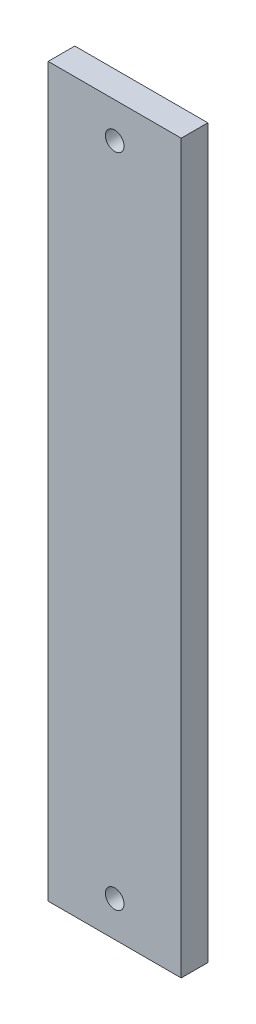
from build123d import *

# Parameters (mm, degrees)
SKETCH1_W                      = 150
SKETCH1_H                      = 820
BOSS_EXTRUDE1_DEPTH            = 30
M24_THREADED_HOLE1_D           = 21
M24_THREADED_HOLE1_ON_FACE_2_D = 21


with BuildPart() as part:
    # Sketch1 → Boss-Extrude1 (new body)
    with BuildSketch(Plane.XY):
        with Locations((75, 410)):
            Rectangle(SKETCH1_W, SKETCH1_H)
    extrude(amount=BOSS_EXTRUDE1_DEPTH)

    # M24 Threaded hole1 (through all)
    with Locations(Plane(origin=(75, 780, 30), x_dir=(1, 0, 0), z_dir=(0, 0, 1))):
        with Locations((0, 0), (0, -740)):
            Hole(M24_THREADED_HOLE1_D / 2)

    # M24 Threaded hole1 on face 2 (through all)
    with Locations(Plane(origin=(283.451995804, 183.295208972, 0), x_dir=(1, 0, 0), z_dir=(0, 0, 1))):
        with Locations((0, 0)):
            Hole(M24_THREADED_HOLE1_ON_FACE_2_D / 2)


solid = part.part
